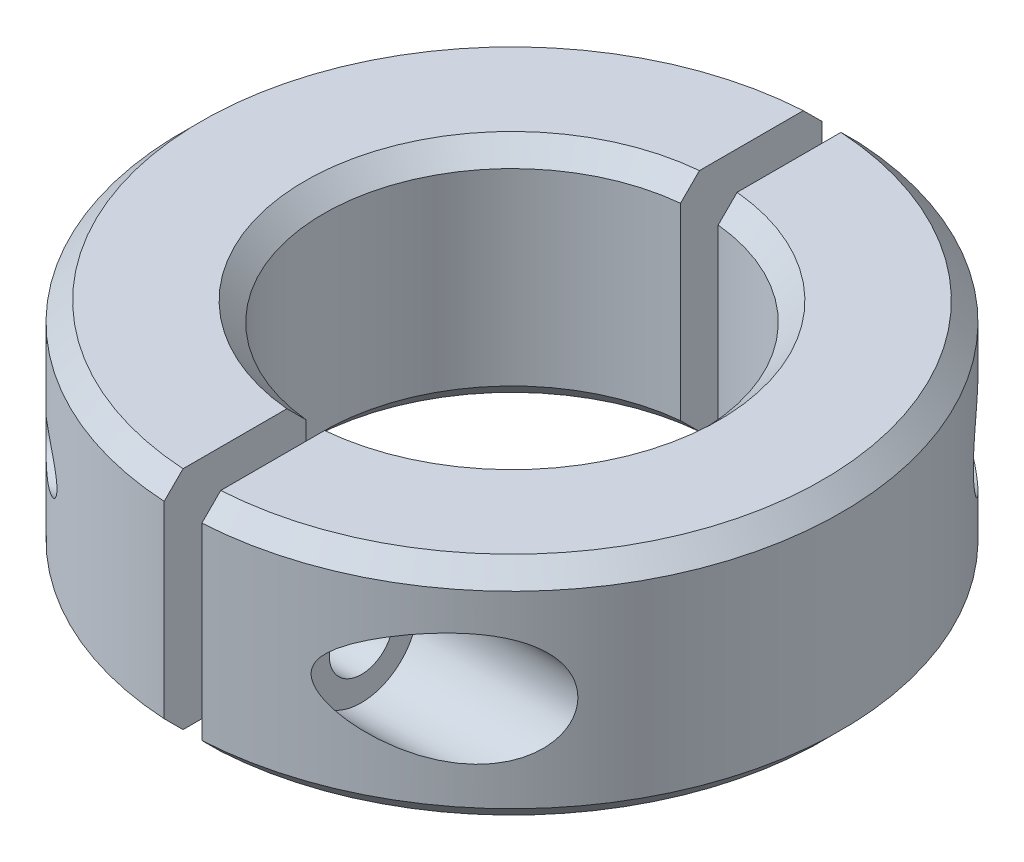
SolidWorks part; units mm, degrees
ref_plane "前视基准面" through (0, 0, 0) normal (0, 0, 1) x (1, 0, 0)
ref_plane "上视基准面" through (0, 0, 0) normal (0, 1, 0) x (1, 0, 0)
ref_plane "右视基准面" through (0, 0, 0) normal (1, 0, 0) x (0, 0, -1)
sketch "草图1" plane through (0, 0, 0) normal (0, 1, 0) x (1, 0, 0)
  circle A0 centre (0, 0) radius 17.5
  circle A1 centre (0, 0) radius 10
  dimension "D1" = 20
  dimension "D2" = 35
extrude "凸台-拉伸1" add sketch "草图1" along normal mid plane 12
chamfer "倒角1" distance 1 angle 45 4 edges at (0, -6, 10) (0, -6, 17.5) (0, 6, 10) (0, 6, 17.5)
sketch "草图2" plane through (0, 6, 0) normal (0, 1, 0) x (1, 0, 0)
  line L1 (-1, -20) -> (1, -20)
  line L2 (-1, -20) -> (-1, 20)
  line L3 (-1, 20) -> (1, 20)
  line L4 (1, -20) -> (1, 20)
  line L5 (-1, -20) -> (1, 20) construction
  line L6 (-1, 20) -> (1, -20) construction
  point P0 (0, 0)
  dimension "D1" = 2
  dimension "D2" = 40
extrude "切除-拉伸1" cut sketch "草图2" against normal through all
ref_plane "基准面1" through (17.5, 0, 0) normal (1, 0, 0) x (0, 0, -1)
sketch "草图5" plane through (17.5, 0, 0) normal (1, 0, 0) x (0, 0, -1)
  line L0 (0, 0) -> (0, 11.8278) construction
  point P0 (13.5, 0)
  dimension "D1" = 13.5
hole_wizard "M3 六角圆柱头螺钉的柱形沉头孔1" positions "草图5" profile "草图6" counterbore size "M3" standard "GB"
sketch "草图6" plane through (17.5, 0, -13.5) normal (0, 1, 0) x (0, 0, -1)
  line L0 (0, 0) -> (0, 17.5215)
  line L1 (0, 17.5215) -> (1.7, 16.5)
  line L2 (1.7, 16.5) -> (1.7, 12)
  line L3 (1.7, 12) -> (3, 12)
  line L4 (3, 12) -> (3, 0)
  line L5 (3, 0) -> (0, 0)
  line L10 (0, 17.5215) -> (-1.7, 16.5) construction
  line L11 (0, -6.35) -> (0, 107.95) construction
  dimension "孔直径" = 3.4
  dimension "孔深度" = 16.5
  dimension "柱形沉头孔直径" = 6
  dimension "柱形沉头孔深度" = 12
  dimension "导头角度" = 118
sketch "草图10" plane through (-1, 0, 0) normal (1, 0, 0) x (0, 0, -1)
  point P0 (13.5, 0)
hole_wizard "M3 螺纹孔1" positions "草图10" profile "草图11" tap size "M3" standard "GB" end condition through all
sketch "草图11" plane through (-1, 0, -13.5) normal (0, 1, 0) x (0, 0, -1)
  line L0 (0, 0) -> (0, 16.5)
  line L1 (0, 16.5) -> (1.25, 16.5)
  line L2 (1.25, 16.5) -> (1.25, 0)
  line L5 (1.25, 0) -> (0, 0)
  line L11 (0, -6.35) -> (0, 107.95) construction
  dimension "通孔螺纹孔钻头直径" = 2.5
  dimension "通孔螺纹孔钻头深度" = 16.5
cosmetic thread "孔螺纹线1" parameters "D2"=3
mirror "镜向1" about plane through (0, 0, 0) normal (0, 0, 1) of "M3 六角圆柱头螺钉的柱形沉头孔1", "M3 螺纹孔1"
